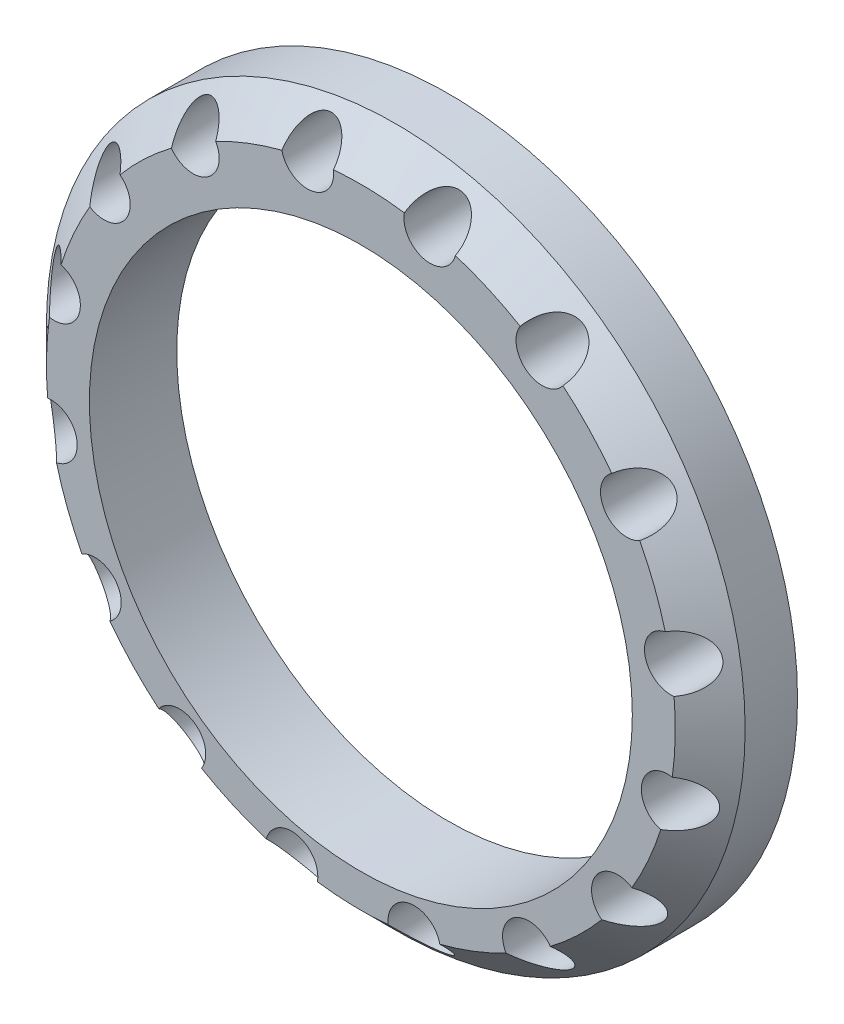
from build123d import *

# Parameters (mm, degrees)
SKETCH1_R           = 20
SKETCH1_R_2         = 15.541192726
BOSS_EXTRUDE1_DEPTH = 5
CHAMFER1_SIZE       = 2
SKETCH2_R           = 1.5
CUT_EXTRUDE1_DEPTH  = 86.879372487


with BuildPart() as part:
    # Sketch1 → Boss-Extrude1 (new body)
    with BuildSketch(Plane.XY):
        with Locations((20, 55.830512452)):
            Circle(SKETCH1_R)
        with Locations((20, 55.289319726)):
            Circle(SKETCH1_R_2, mode=Mode.SUBTRACT)
    extrude(amount=BOSS_EXTRUDE1_DEPTH)

    # Chamfer1
    chamfer1_edges = [part.edges().sort_by_distance(p)[0] for p in [
        (0, 55.830512452, 5),
    ]]
    chamfer(chamfer1_edges, length=CHAMFER1_SIZE)

    # Sketch2 → Cut-Extrude1 (cut, through all)
    with BuildSketch(Plane.XY.offset(5)):
        with Locations((10.388397973, 71.049484377)):
            Circle(SKETCH2_R)
        with Locations((16.944086026, 73.569209974)):
            Circle(SKETCH2_R)
        with Locations((23.96500928, 73.388379674)):
            Circle(SKETCH2_R)
        with Locations((30.382295814, 70.534523253)):
            Circle(SKETCH2_R)
        with Locations((35.218971926, 65.442114479)):
            Circle(SKETCH2_R)
        with Locations((37.738697522, 58.886426426)):
            Circle(SKETCH2_R)
        with Locations((37.557867223, 51.865503172)):
            Circle(SKETCH2_R)
        with Locations((34.704010801, 45.448216638)):
            Circle(SKETCH2_R)
        with Locations((29.611602027, 40.611540526)):
            Circle(SKETCH2_R)
        with Locations((23.055913974, 38.09181493)):
            Circle(SKETCH2_R)
        with Locations((16.03499072, 38.272645229)):
            Circle(SKETCH2_R)
        with Locations((9.617704186, 41.126501651)):
            Circle(SKETCH2_R)
        with Locations((4.781028074, 46.218910425)):
            Circle(SKETCH2_R)
        with Locations((2.261302478, 52.774598478)):
            Circle(SKETCH2_R)
        with Locations((2.442132777, 59.795521732)):
            Circle(SKETCH2_R)
        with Locations((5.295989199, 66.212808266)):
            Circle(SKETCH2_R)
    extrude(amount=-CUT_EXTRUDE1_DEPTH, mode=Mode.SUBTRACT)


solid = part.part
